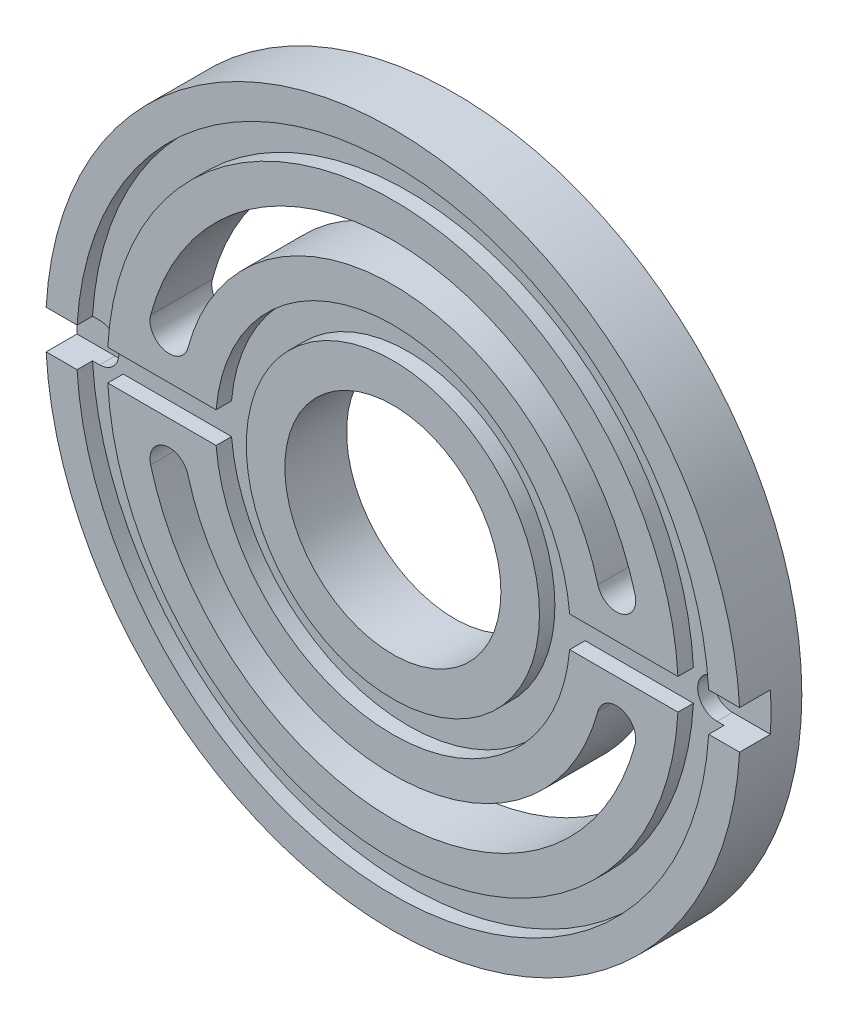
from build123d import *

# Parameters (mm, degrees)
SKETCH1_R           = 45
SKETCH1_R_2         = 14
BOSS_EXTRUDE1_DEPTH = 8
SKETCH2_R           = 41
SKETCH2_R_2         = 37
SKETCH2_R_3         = 23
SKETCH2_R_4         = 19
CUT_EXTRUDE1_DEPTH  = 2
CUT_EXTRUDE2_DEPTH  = 100
CUT_EXTRUDE3_DEPTH  = 4
CUT_EXTRUDE4_DEPTH  = 2


with BuildPart() as part:
    # Sketch1 → Boss-Extrude1 (new body)
    with BuildSketch(Plane.XY):
        Circle(SKETCH1_R)
        Circle(SKETCH1_R_2, mode=Mode.SUBTRACT)
    extrude(amount=BOSS_EXTRUDE1_DEPTH)

    # Sketch2 → Cut-Extrude1 (cut)
    # profile 1 of 4: a face of its own
    with BuildSketch(Plane.XY.offset(8)):
        Circle(SKETCH2_R)
        Circle(SKETCH2_R_2, mode=Mode.SUBTRACT)
    # profile 2 of 4: a face of its own
    with BuildSketch(Plane.XY.offset(8)):
        Circle(SKETCH2_R_3)
        Circle(SKETCH2_R_4, mode=Mode.SUBTRACT)
    # profile 3 of 4: a face of its own
    with BuildSketch(Plane.XY.offset(8)):
        with BuildLine():
            ThreePointArc((31.392589354, 8.411618966), (0, 32.5), (-31.392589354, 8.411618966))
            ThreePointArc((-31.392589354, 8.411618966), (-29.624822401, 5.349756787), (-26.562960223, 7.11752374))
            ThreePointArc((-26.562960223, 7.11752374), (0, 27.5), (26.562960223, 7.11752374))
            ThreePointArc((26.562960223, 7.11752374), (29.624822401, 5.349756787), (31.392589354, 8.411618966))
        make_face()
    # profile 4 of 4: a face of its own
    with BuildSketch(Plane.XY.offset(8)):
        with BuildLine():
            ThreePointArc((-31.392589354, -8.411618966), (-29.624822401, -5.349756787), (-26.562960223, -7.11752374))
            ThreePointArc((-26.562960223, -7.11752374), (0, -27.5), (26.562960223, -7.11752374))
            ThreePointArc((26.562960223, -7.11752374), (29.624822401, -5.349756787), (31.392589354, -8.411618966))
            ThreePointArc((31.392589354, -8.411618966), (0, -32.5), (-31.392589354, -8.411618966))
        make_face()
    extrude(amount=-CUT_EXTRUDE1_DEPTH, mode=Mode.SUBTRACT)

    # Sketch3 → Cut-Extrude2 (cut)
    with BuildSketch(Plane.XY.offset(6)):
        with BuildLine():
            ThreePointArc((31.392589354, 8.411618966), (0, 32.5), (-31.392589354, 8.411618966))
            ThreePointArc((-31.392589354, 8.411618966), (-29.624822401, 5.349756787), (-26.562960223, 7.11752374))
            ThreePointArc((-26.562960223, 7.11752374), (0, 27.5), (26.562960223, 7.11752374))
            ThreePointArc((26.562960223, 7.11752374), (29.624822401, 5.349756787), (31.392589354, 8.411618966))
        make_face()
        with BuildLine():
            ThreePointArc((-26.562960223, -7.11752374), (-29.624822401, -5.349756787), (-31.392589354, -8.411618966))
            ThreePointArc((-31.392589354, -8.411618966), (0, -32.5), (31.392589354, -8.411618966))
            ThreePointArc((31.392589354, -8.411618966), (29.624822401, -5.349756787), (26.562960223, -7.11752374))
            ThreePointArc((26.562960223, -7.11752374), (0, -27.5), (-26.562960223, -7.11752374))
        make_face()
    extrude(amount=-CUT_EXTRUDE2_DEPTH, mode=Mode.SUBTRACT)

    # Sketch4<3> → Cut-Extrude3 (cut)
    with BuildSketch(Plane.XY.offset(8)):
        with BuildLine():
            Line((-45, -2.5), (-40, -2.5))
            ThreePointArc((-40, -2.5), (-37.5, 0), (-40, 2.5))
            Line((-40, 2.5), (-45, 2.5))
            ThreePointArc((-45, 2.5), (-47.5, 0), (-45, -2.5))
        make_face()
        with BuildLine():
            ThreePointArc((40, -2.5), (37.5, 0), (40, 2.5))
            Line((40, 2.5), (45, 2.5))
            ThreePointArc((45, 2.5), (47.5, 0), (45, -2.5))
            Line((45, -2.5), (40, -2.5))
        make_face()
    extrude(amount=-CUT_EXTRUDE3_DEPTH, mode=Mode.SUBTRACT)

    # 草图4<3> → Cut-Extrude4 (cut)
    with BuildSketch(Plane.XY.offset(8)):
        with BuildLine():
            Line((22.912878475, -2), (36.945906404, -2))
            ThreePointArc((36.945906404, -2), (36.986474129, -1.000365698), (37, 0))
            ThreePointArc((37, 0), (36.986474129, 1.000365698), (36.945906404, 2))
            Line((36.945906404, 2), (22.912878475, 2))
            ThreePointArc((22.912878475, 2), (22.978209296, 1.00094832), (23, 0))
            ThreePointArc((23, 0), (22.978209296, -1.00094832), (22.912878475, -2))
        make_face()
        with BuildLine():
            ThreePointArc((-36.945906404, 2), (-37, 0), (-36.945906404, -2))
            Line((-36.945906404, -2), (-22.912878475, -2))
            ThreePointArc((-22.912878475, -2), (-23, 0), (-22.912878475, 2))
            Line((-22.912878475, 2), (-36.945906404, 2))
        make_face()
        with BuildLine():
            Line((22.912878475, -2), (36.945906404, -2))
            ThreePointArc((36.945906404, -2), (36.986474129, -1.000365698), (37, 0))
            ThreePointArc((37, 0), (36.986474129, 1.000365698), (36.945906404, 2))
            Line((36.945906404, 2), (22.912878475, 2))
            ThreePointArc((22.912878475, 2), (22.978209296, 1.00094832), (23, 0))
            ThreePointArc((23, 0), (22.978209296, -1.00094832), (22.912878475, -2))
        make_face()
        with BuildLine():
            ThreePointArc((-36.945906404, 2), (-37, 0), (-36.945906404, -2))
            Line((-36.945906404, -2), (-22.912878475, -2))
            ThreePointArc((-22.912878475, -2), (-23, 0), (-22.912878475, 2))
            Line((-22.912878475, 2), (-36.945906404, 2))
        make_face()
    extrude(amount=-CUT_EXTRUDE4_DEPTH, mode=Mode.SUBTRACT)


solid = part.part
